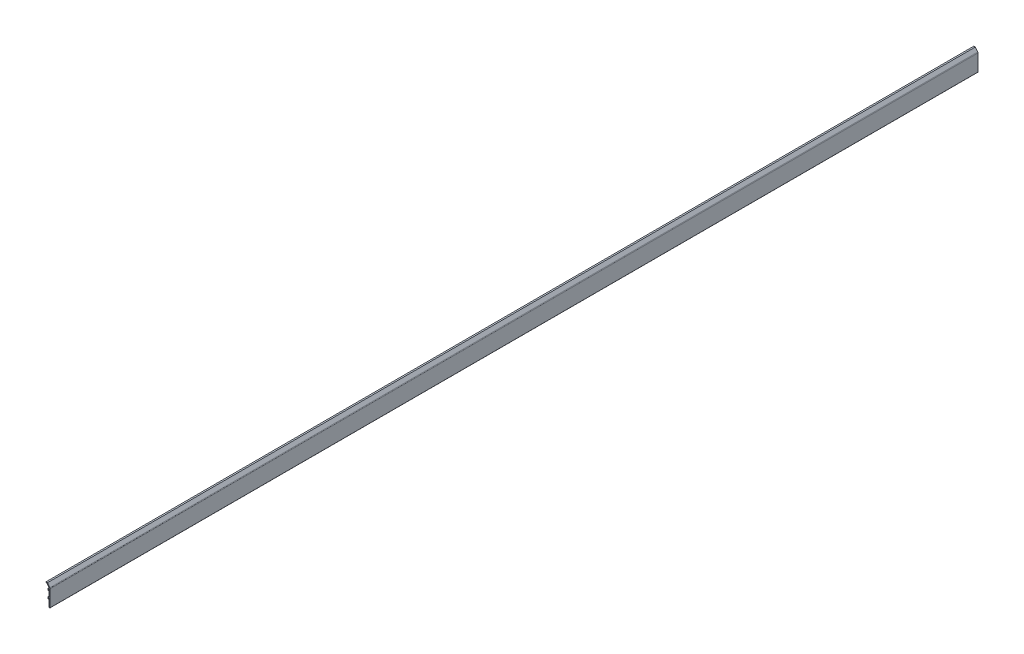
from build123d import *

# Parameters (mm, degrees)
EXTRUDE_1_DEPTH = 1058


with BuildPart() as part:
    # 草图2 → 凸台-拉伸1 (new, symmetric)
    with BuildSketch(Plane.XY):
        with BuildLine():
            Line((-2.699712502, 32.249908534), (-2.499724552, 32.249908534))
            ThreePointArc((-2.499724552, 32.249908534), (-2.075486045, 32.425633877), (-1.899760702, 32.849872384))
            Line((-1.899760702, 32.849872384), (-1.899760702, 36.12977276))
            ThreePointArc((-1.899760702, 36.12977276), (-1.864615633, 36.214620461), (-1.779767932, 36.24976553))
            Line((-1.779767932, 36.24976553), (0, 36.24976553))
            Line((0, 36.24976553), (0.000764104, 20.44942184))
            Line((0.000764104, 20.44942184), (-2.498960448, 20.44942184))
            ThreePointArc((-2.498960448, 20.44942184), (-2.781786119, 20.332271611), (-2.898936348, 20.04944594))
            Line((-2.898936348, 20.04944594), (-2.898936348, 15.649613044))
            ThreePointArc((-2.898936348, 15.649613044), (-2.840361233, 15.508200208), (-2.698948398, 15.449625094))
            Line((-2.698948398, 15.449625094), (-2.498960448, 15.449625094))
            ThreePointArc((-2.498960448, 15.449625094), (-2.074721941, 15.625350437), (-1.898996598, 16.049588944))
            Line((-1.898996598, 16.049588944), (-1.898996598, 19.32948932))
            ThreePointArc((-1.898996598, 19.32948932), (-1.863851529, 19.414337021), (-1.779003828, 19.44948209))
            Line((-1.779003828, 19.44948209), (0.000764104, 19.44948209))
            Line((0.000764104, 19.44948209), (0, 0))
            Line((0, 0), (1.5, 0))
            ThreePointArc((1.5, 0), (1.853553391, 0.146446609), (2, 0.5))
            Line((2, 0.5), (2, 38.058011928))
            ThreePointArc((2, 38.058011928), (1.844147591, 39.012383177), (1.392783679, 39.867593721))
            Line((1.392783679, 39.867593721), (-4, 46.998393128))
            Line((-4, 46.998393128), (-7.4, 46.998393128))
            Line((-7.4, 46.998393128), (-7.4, 45.998393128))
            Line((-7.4, 45.998393128), (-5.751273316, 45.998393128))
            Line((-5.751273316, 45.998393128), (-0.607216321, 39.196481397))
            ThreePointArc((-0.607216321, 39.196481397), (-0.155852409, 38.341270854), (0, 37.386899605))
            Line((0, 37.386899605), (0, 37.24970528))
            Line((0, 37.24970528), (-2.499724552, 37.24970528))
            ThreePointArc((-2.499724552, 37.24970528), (-2.782550223, 37.132555051), (-2.899700452, 36.84972938))
            Line((-2.899700452, 36.84972938), (-2.899700452, 32.449896484))
            ThreePointArc((-2.899700452, 32.449896484), (-2.841125337, 32.308483648), (-2.699712502, 32.249908534))
        make_face()
    extrude(amount=EXTRUDE_1_DEPTH, both=True)


solid = part.part
